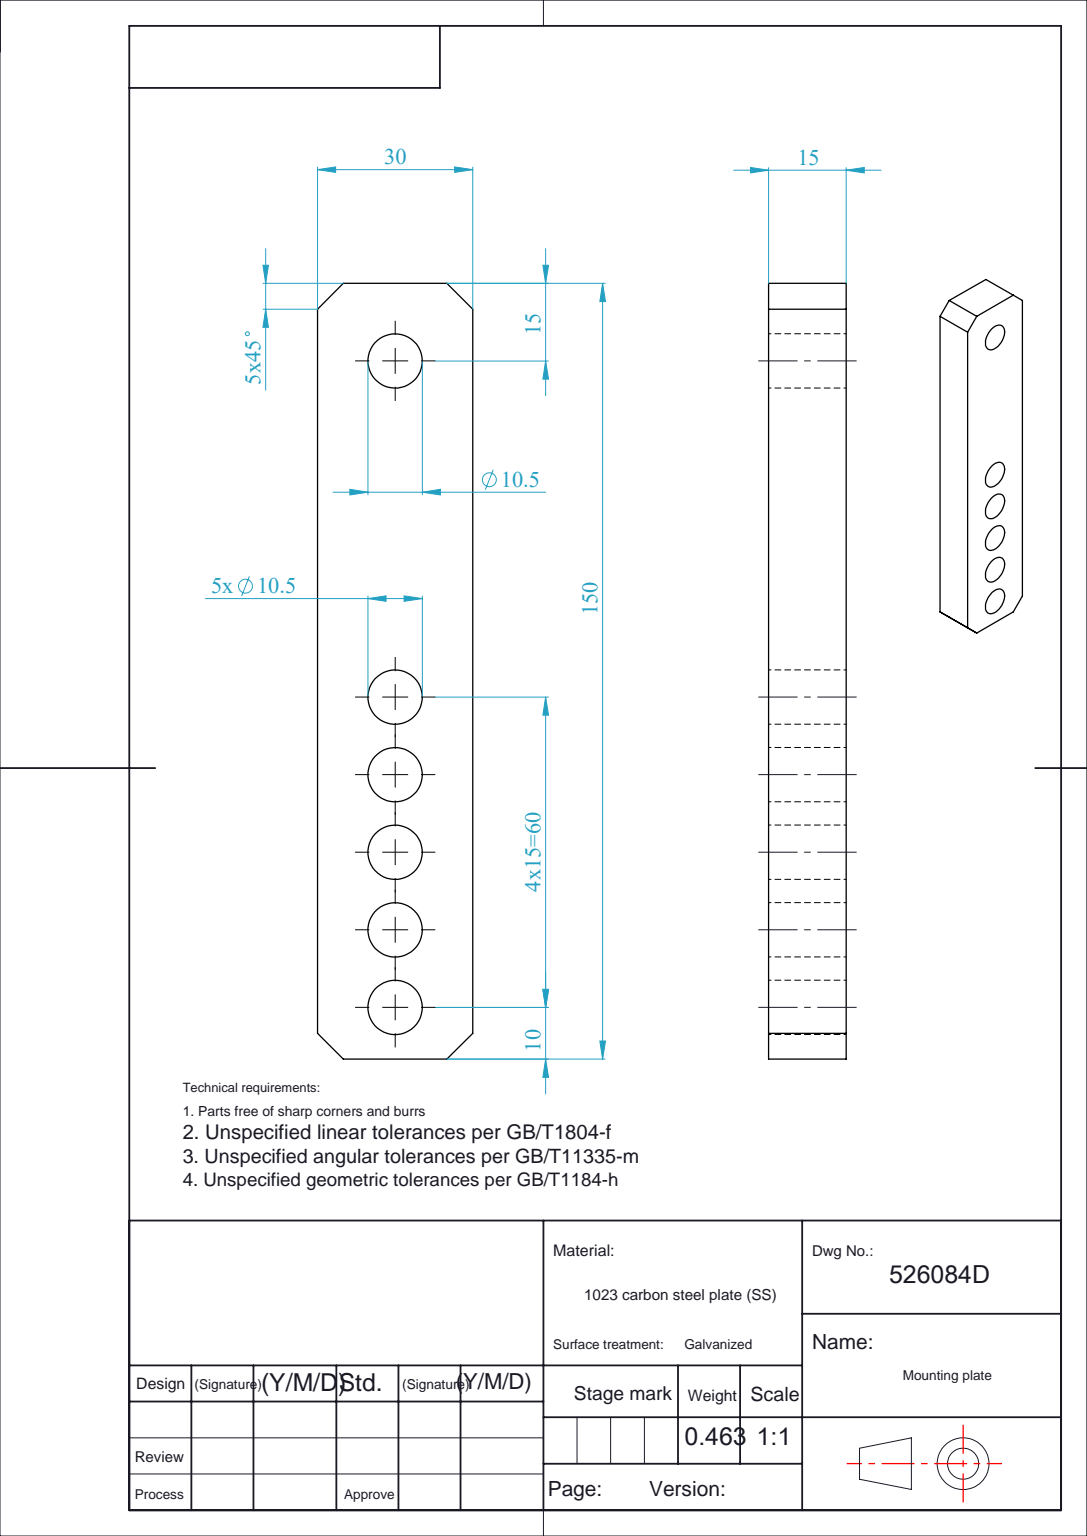
from build123d import *

# Parameters (mm, degrees)
SKETCH1_W           = 30
SKETCH1_H           = 150
BOSS_EXTRUDE1_DEPTH = 15
CHAMFER1_SIZE       = 5
SKETCH2_R           = 5.25
CUT_EXTRUDE1_DEPTH  = 43


with BuildPart() as part:
    # Sketch1 → Boss-Extrude1 (new body)
    with BuildSketch(Plane.XY):
        Rectangle(SKETCH1_W, SKETCH1_H)
    extrude(amount=BOSS_EXTRUDE1_DEPTH)

    # Chamfer1
    chamfer1_edges = [part.edges().sort_by_distance(p)[0] for p in [
        (15, -75, 7.5),
        (-15, -75, 7.5),
        (-15, 75, 7.5),
        (15, 75, 7.5),
    ]]
    chamfer(chamfer1_edges, length=CHAMFER1_SIZE)

    # Sketch2 → Cut-Extrude1 (cut)
    with BuildSketch(Plane.XY.offset(15)):
        with Locations((0, 60)):
            Circle(SKETCH2_R)
        with Locations((0, -5)):
            Circle(SKETCH2_R)
        with Locations((0, -20)):
            Circle(SKETCH2_R)
        with Locations((0, -35)):
            Circle(SKETCH2_R)
        with Locations((0, -50)):
            Circle(SKETCH2_R)
        with Locations((0, -65)):
            Circle(SKETCH2_R)
    extrude(amount=-CUT_EXTRUDE1_DEPTH, mode=Mode.SUBTRACT)


solid = part.part
